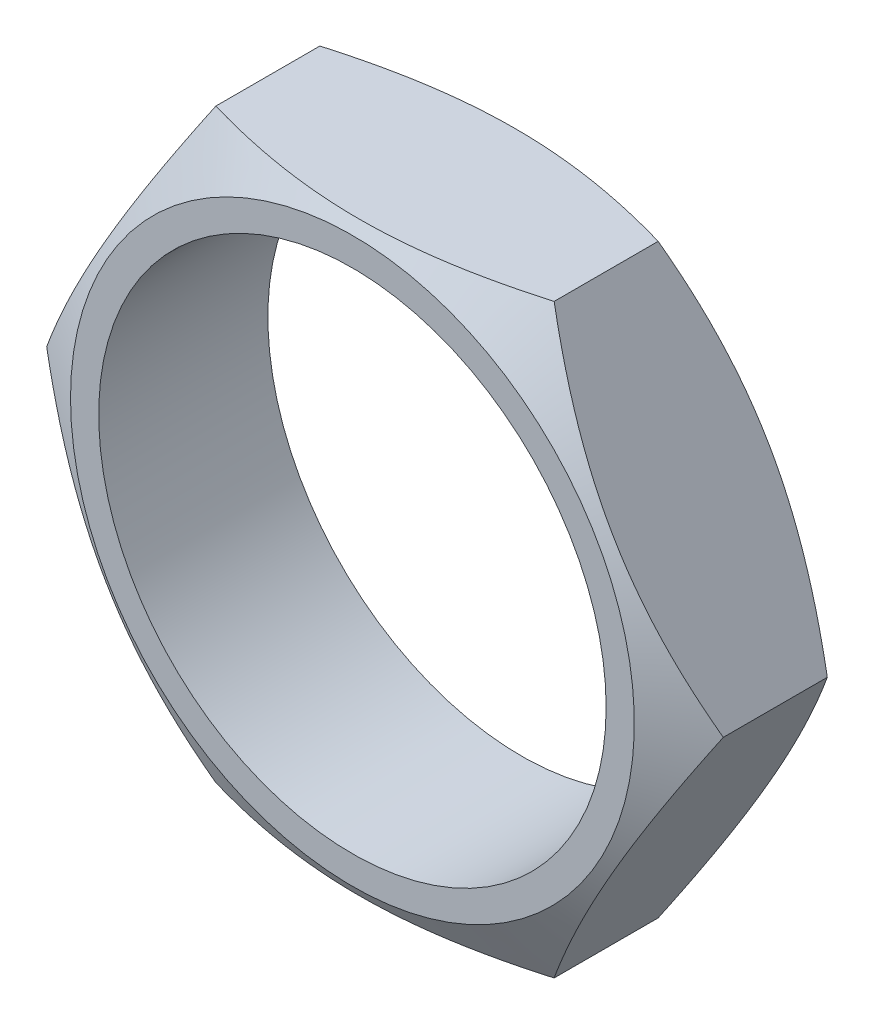
SolidWorks part; units mm, degrees
ref_plane "前视基准面" through (0, 0, 0) normal (0, 0, 1) x (1, 0, 0)
ref_plane "上视基准面" through (0, 0, 0) normal (0, 1, 0) x (1, 0, 0)
ref_plane "右视基准面" through (0, 0, 0) normal (1, 0, 0) x (0, 0, -1)
sketch "草图1" plane through (0, 0, 0) normal (0, 0, 1) x (1, 0, 0)
  line L1 (24, 0) -> (12, 20.7846)
  line L2 (12, 20.7846) -> (-12, 20.7846)
  line L3 (-12, 20.7846) -> (-24, 0)
  line L4 (-24, 0) -> (-12, -20.7846)
  line L5 (-12, -20.7846) -> (12, -20.7846)
  line L6 (12, -20.7846) -> (24, 0)
  circle A0 centre (0, 0) radius 18
  dimension "D1" = 36
  dimension "D2" = 48
extrude "凸台-拉伸1" add sketch "草图1" along normal blind 12
cosmetic thread "装饰螺纹线1" parameters "D2"=39
sketch "草图2" plane through (0, 0, 0) normal (0, 1, 0) x (1, 0, 0)
  line L0 (-24, 0) -> (-24, -2.3094)
  line L1 (-24, -12) -> (-24, 0) construction
  line L2 (-24, -2.3094) -> (-20, 0)
  line L3 (-12, 0) -> (-24, 0) construction
  line L4 (-20, 0) -> (-24, 0)
  line L5 (-24, -12) -> (-24, -9.6906)
  line L6 (-24, -9.6906) -> (-20, -12)
  line L7 (-12, -12) -> (-24, -12) construction
  line L8 (-24, -12) -> (-20, -12)
  line L9 (0, 5.9718) -> (0, -14.1606) construction
  dimension "D1" = 4
  dimension "D2" = 30
  dimension "D3" = 4
  dimension "D4" = 30
revolve "切除-旋转1" cut sketch "草图2" angle 360 about L9
